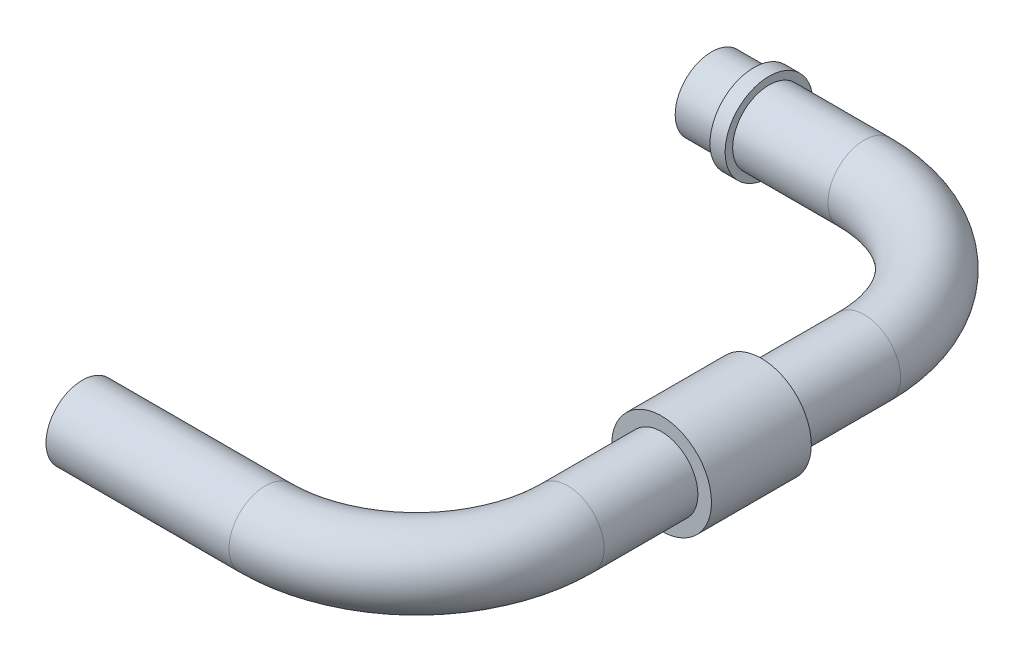
SolidWorks part; units mm, degrees
ref_plane "Front" through (0, 0, 0) normal (0, 0, 1) x (1, 0, 0)
ref_plane "Top" through (0, 0, 0) normal (0, 1, 0) x (1, 0, 0)
ref_plane "Right" through (0, 0, 0) normal (1, 0, 0) x (0, 0, -1)
sketch "草图1" plane through (0, 0, 0) normal (0, 1, 0) x (1, 0, 0)
  line L0 (0, 0) -> (60.5, 0)
  line L1 (110.5, 50) -> (110.5, 148)
  line L2 (60.5, 198) -> (10, 198)
  arc A0 (60.5, 0) -> (110.5, 50) centre (60.5, 50) ccw
  arc A1 (110.5, 148) -> (60.5, 198) centre (60.5, 148) ccw
  point P7 (110.5, 0)
  point P10 (110.5, 198)
  dimension "D4" = 50
  dimension "D1" = 198
  dimension "D2" = 110.5
  dimension "D3" = 100.5
sweep "扫描1" add path "草图1" circular profile diameter 24 parameters "D3"=24
sketch "草图14" plane through (10, 0, 0) normal (-1, 0, 0) x (0, 0, 1)
  circle A0 centre (-198, 0) radius 14.5
  dimension "D1" = 29
extrude "凸台-拉伸1" add sketch "草图14" against normal blind 5 from offset 14 offset against normal yes
ref_plane "基准面1" through (0, 0, -97.5) normal (0, 0, 1) x (1, 0, 0)
sketch "草图16" plane through (0, 0, -97.5) normal (0, 0, 1) x (1, 0, 0)
  circle A0 centre (110.5, 0) radius 16.5
  dimension "D1" = 33
extrude "凸台-拉伸2" add sketch "草图16" along normal mid plane 33
